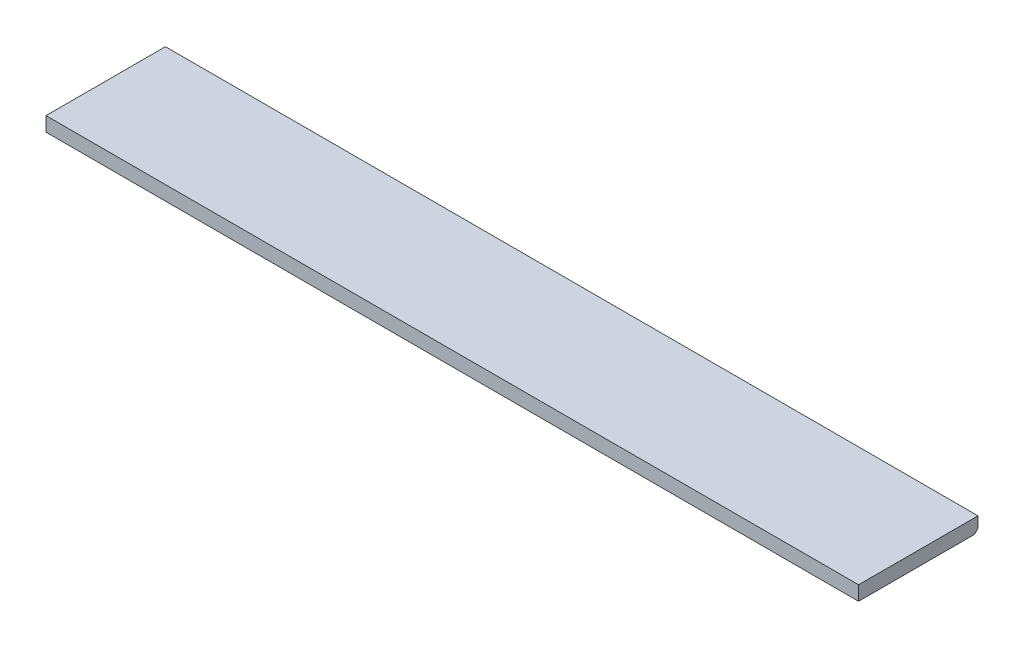
from build123d import *

# Parameters (mm, degrees)
SKETCH_1_W      = 2266
SKETCH_1_H      = 333
EXTRUDE_1_DEPTH = 40
CHAMFER_1_SIZE  = 10


with BuildPart() as part:
    # 草图1 → 凸台-拉伸1 (new body)
    with BuildSketch(Plane(origin=(0, 0, 0), x_dir=(1, 0, 0), z_dir=(0, 1, 0))):
        Rectangle(SKETCH_1_W, SKETCH_1_H)
    extrude(amount=EXTRUDE_1_DEPTH)

    # 倒角1
    chamfer_1_edges = [part.edges().sort_by_distance(p)[0] for p in [
        (0, 0, -166.5),
    ]]
    chamfer(chamfer_1_edges, length=CHAMFER_1_SIZE)


solid = part.part
